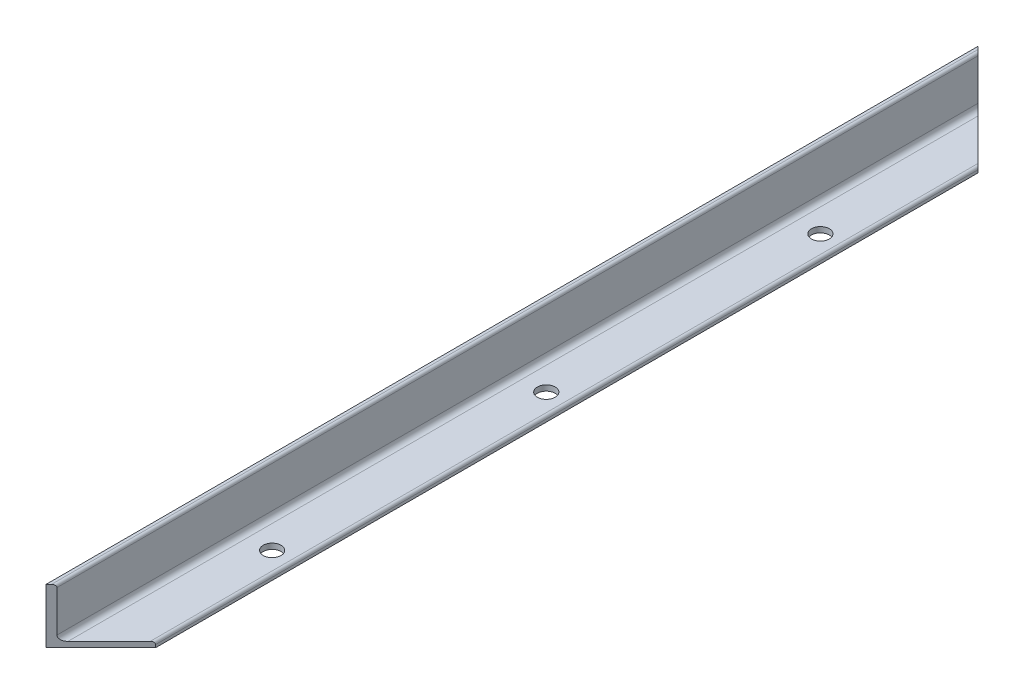
SolidWorks part; units mm, degrees
material "等边XRC0×4/Q235A"
ref_plane "Front Plane" through (0, 0, 0) normal (0, 0, 1) x (1, 0, 0)
ref_plane "Top Plane" through (0, 0, 0) normal (0, 1, 0) x (1, 0, 0)
ref_plane "Right Plane" through (0, 0, 0) normal (1, 0, 0) x (0, 0, -1)
sketch "Sketch1" plane through (0, 0, 0) normal (0, 0, 1) x (1, 0, 0)
  line L0 (0, 40) -> (0, 0)
  line L1 (0, 0) -> (40, 0)
  line L2 (40, 0) -> (40, 2)
  line L3 (38, 4) -> (8, 4)
  line L4 (4, 8) -> (4, 38)
  line L5 (2, 40) -> (0, 40)
  arc A0 (8, 4) -> (4, 8) centre (8, 8) cw
  arc A1 (40, 2) -> (38, 4) centre (38, 2) ccw
  arc A2 (4, 38) -> (2, 40) centre (2, 38) ccw
  point P11 (40, 4)
  dimension "D5" = 4
  dimension "D6" = 2
  dimension "D1" = 40
  dimension "D2" = 40
  dimension "D3" = 4
  dimension "D4" = 4
extrude "Boss-Extrude1" add sketch "Sketch1" along normal blind 680
sketch "Sketch2" plane through (0, 4, 0) normal (0, 1, 0) x (1, 0, 0)
  line L0 (0, 0) -> (40, -40)
  line L1 (40, -680) -> (40, 0) construction
  line L2 (40, -40) -> (40, 0)
  line L3 (40, 0) -> (0, 0)
  line L4 (0, -680) -> (40, -680)
  line L5 (40, -680) -> (40, -640)
  line L6 (40, -640) -> (0, -680)
  dimension "D1" = 45
  dimension "D2" = 45
extrude "Cut-Extrude1" cut sketch "Sketch2" against normal through all both and the other way through all
sketch "Sketch3" plane through (0, 4, 0) normal (0, 1, 0) x (1, 0, 0)
  line L0 (40, -640) -> (40, -40) construction
  circle A0 centre (25, -140) radius 6.5
  circle A1 centre (25, -340) radius 6.5
  circle A2 centre (25, -540) radius 6.5
  dimension "D1" = 13
  dimension "D2" = 15
  dimension "D3" = 140
  dimension "D4" = 3
extrude "Cut-Extrude2" cut sketch "Sketch3" against normal blind 10
